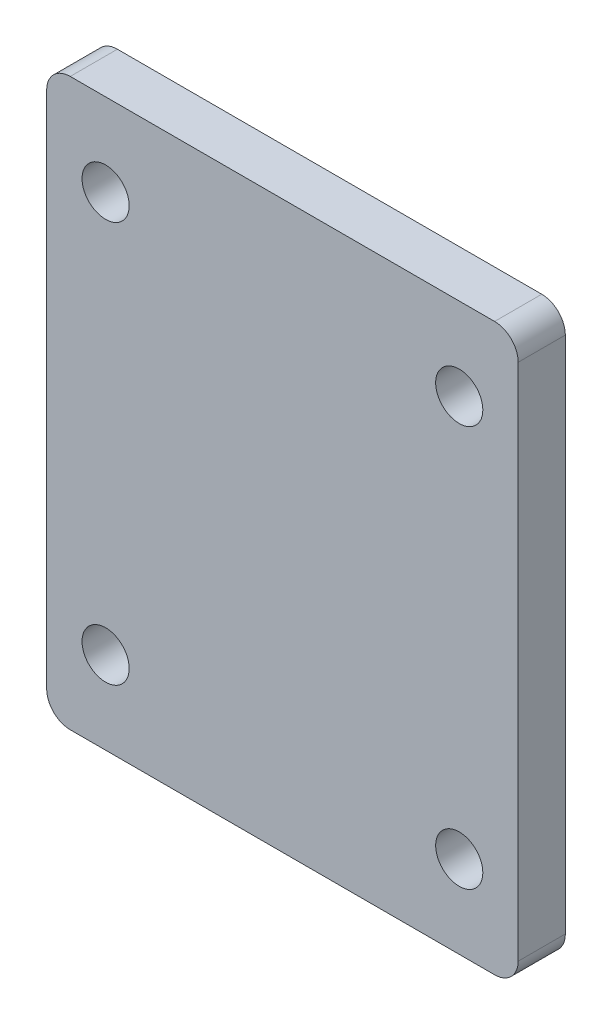
SolidWorks part; units mm, degrees
ref_plane "Front Plane" through (0, 0, 0) normal (0, 0, 1) x (1, 0, 0)
ref_plane "Top Plane" through (0, 0, 0) normal (0, 1, 0) x (1, 0, 0)
ref_plane "Right Plane" through (0, 0, 0) normal (1, 0, 0) x (0, 0, -1)
sketch "Sketch1" plane through (0, 0, 0) normal (0, 0, 1) x (1, 0, 0)
  line L0 (50, 7.4354) -> (50, -134.4805) construction
  line L1 (5, 0) -> (95, 0)
  line L2 (0, -5) -> (0, -115)
  line L3 (5, -120) -> (95, -120)
  line L4 (100, -5) -> (100, -115)
  line L5 (0, 0) -> (100, -120) construction
  line L6 (0, -120) -> (100, 0) construction
  line L7 (-14.9795, -60) -> (109.6094, -60) construction
  arc A0 (0, -115) -> (5, -120) centre (5, -115) ccw
  arc A1 (95, -120) -> (100, -115) centre (95, -115) ccw
  arc A2 (100, -5) -> (95, 0) centre (95, -5) ccw
  arc A3 (0, -5) -> (5, 0) centre (5, -5) cw
  circle A4 centre (12.5, -17.5) radius 5
  circle A5 centre (87.5, -17.5) radius 5
  circle A6 centre (87.5, -102.5) radius 5
  circle A7 centre (12.5, -102.5) radius 5
  point P4 (50, -60)
  dimension "D3" = 5
  dimension "D4" = 75
  dimension "D8" = 10
  dimension "D1" = 100
  dimension "D2" = 120
  dimension "D5" = 85
  dimension "D6" = 37.5
  dimension "D7" = 42.5
extrude "Boss-Extrude1" add sketch "Sketch1" along normal blind 10
